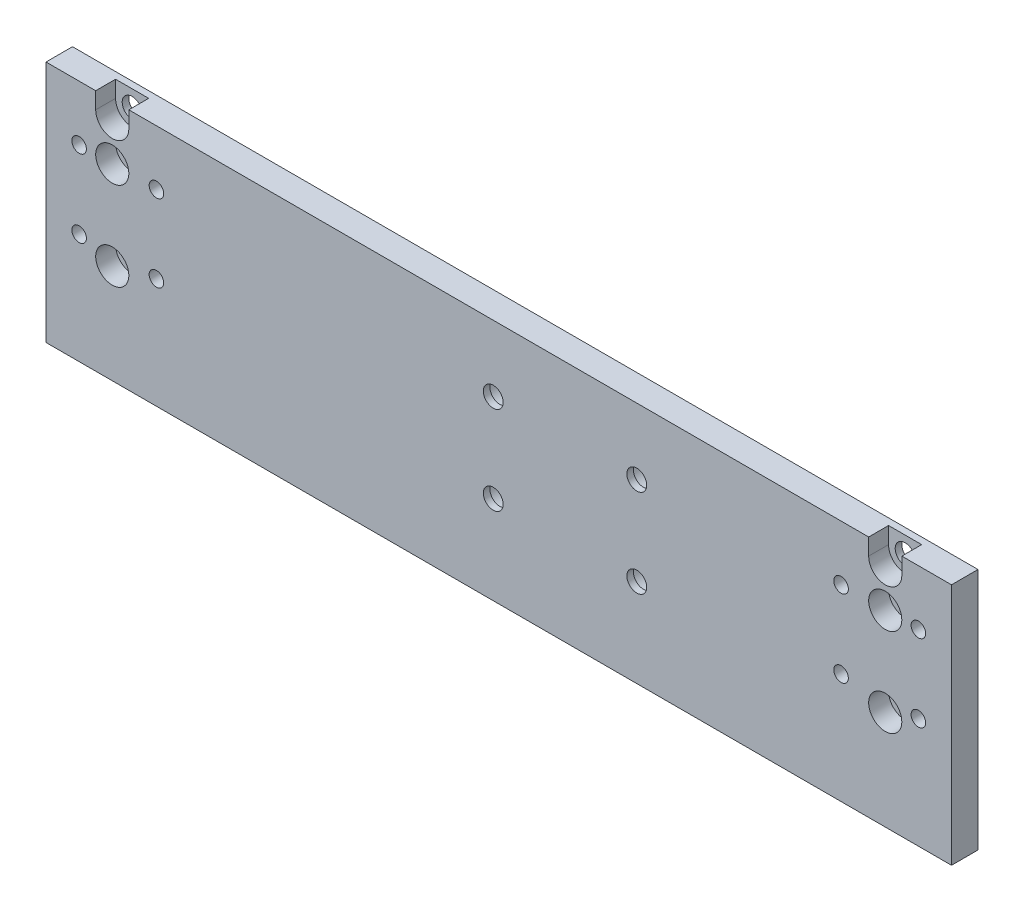
SolidWorks part; units mm, degrees
material "6061 合金"
ref_plane "前视基准面" through (0, 0, 0) normal (0, 0, 1) x (1, 0, 0)
ref_plane "上视基准面" through (0, 0, 0) normal (0, 1, 0) x (1, 0, 0)
ref_plane "右视基准面" through (0, 0, 0) normal (1, 0, 0) x (0, 0, -1)
sketch "草图1" plane through (0, 0, 0) normal (0, 0, 1) x (1, 0, 0)
  line L1 (-205, 55) -> (205, 55)
  line L2 (-205, 55) -> (-205, -55)
  line L3 (-205, -55) -> (205, -55)
  line L4 (205, 55) -> (205, -55)
  line L5 (-205, 55) -> (205, -55) construction
  line L6 (-205, -55) -> (205, 55) construction
  point P0 (0, 0)
  dimension "D1" = 410
  dimension "D2" = 110
extrude "凸台-拉伸1" add sketch "草图1" along normal mid plane 12
hole_wizard "打孔尺寸(%根据)内六角圆柱头螺钉的类型3" positions "3D草图1" profile "草图3" counterbore size "M6" standard "GB"
sketch3d "3D草图1"
  line L1 (205, -55, -6) -> (205, 55, -6) construction
  line L2 (205, 55, -6) -> (-205, 55, -6) construction
  point P0 (190, 30, -6)
  point P2 (155, 30, -6)
  point P4 (190, -5, -6)
  point P6 (155, -5, -6)
  dimension "D1" = 35
  dimension "D2" = 35
  dimension "D3" = 15
  dimension "D4" = 15
  dimension "D5" = 25
  dimension "D6" = 25
  dimension "D7" = 35
  dimension "D8" = 35
sketch "草图3" plane through (190, 30, -6) normal (1, 0, 0) x (0, 1, 0)
  line L0 (0, 0) -> (0, 14.3828)
  line L1 (0, 14.3828) -> (3.3, 12.4)
  line L2 (3.3, 12.4) -> (3.3, 6.8)
  line L3 (3.3, 6.8) -> (5.5, 6.8)
  line L4 (5.5, 6.8) -> (5.5, 0)
  line L5 (5.5, 0) -> (0, 0)
  line L10 (0, 14.3828) -> (-3.3, 12.4) construction
  line L11 (0, -6.35) -> (0, 107.95) construction
  dimension "孔直径" = 6.6
  dimension "孔深度" = 12.4
  dimension "柱形沉头孔直径" = 11
  dimension "柱形沉头孔深度" = 6.8
  dimension "导头角度" = 118
pattern_linear "阵列(线性)1" count 2 spacing 345 along (-1, 0, 0) of "打孔尺寸(%根据)内六角圆柱头螺钉的类型3"
hole_wizard "打孔尺寸(%根据)内六角圆柱头螺钉的类型2" positions "3D草图2" profile "草图4" counterbore size "M8" standard "GB"
sketch3d "3D草图2"
  line L0 (205, 55, -6) -> (-205, 55, -6) construction
  line L1 (-205, -55, -6) -> (205, -55, -6) construction
  line L2 (-205, 55, -6) -> (-205, -55, -6) construction
  point P0 (62.5, 25, -6)
  point P2 (62.5, -15, -6)
  point P4 (-2.5, -15, -6)
  point P6 (-2.5, 25, -6)
  dimension "D1" = 65
  dimension "D2" = 65
  dimension "D3" = 30
  dimension "D4" = 40
  dimension "D5" = 40
  dimension "D6" = 30
  dimension "D7" = 202.5
  dimension "D8" = 202.5
sketch "草图4" plane through (62.5, 25, -6) normal (1, 0, 0) x (0, 1, 0)
  line L0 (0, 0) -> (0, 15.1039)
  line L1 (0, 15.1039) -> (4.5, 12.4)
  line L2 (4.5, 12.4) -> (4.5, 9)
  line L3 (4.5, 9) -> (7.5, 9)
  line L4 (7.5, 9) -> (7.5, 0)
  line L5 (7.5, 0) -> (0, 0)
  line L10 (0, 15.1039) -> (-4.5, 12.4) construction
  line L11 (0, -6.35) -> (0, 107.95) construction
  dimension "孔直径" = 9
  dimension "孔深度" = 12.4
  dimension "柱形沉头孔直径" = 15
  dimension "柱形沉头孔深度" = 9
  dimension "导头角度" = 118
hole_wizard "打孔尺寸(%根据)内六角圆柱头螺钉的类型3" positions "3D草图3" profile "草图5" counterbore size "M8" standard "GB"
sketch3d "3D草图3"
  line L0 (-205, 55, 6) -> (-205, -55, 6) construction
  line L1 (205, 55, 6) -> (-205, 55, 6) construction
  point P4 (-175, 30, 6)
  point P6 (-175, -10, 6)
  dimension "D2" = 30
  dimension "D3" = 30
  dimension "D4" = 40
  dimension "D8" = 25
sketch "草图5" plane through (-175, 30, 6) normal (1, 0, 0) x (0, -1, 0)
  line L0 (0, 0) -> (0, 15.1039)
  line L1 (0, 15.1039) -> (4.5, 12.4)
  line L2 (4.5, 12.4) -> (4.5, 9)
  line L3 (4.5, 9) -> (7.5, 9)
  line L4 (7.5, 9) -> (7.5, 0)
  line L5 (7.5, 0) -> (0, 0)
  line L10 (0, 15.1039) -> (-4.5, 12.4) construction
  line L11 (0, -6.35) -> (0, 107.95) construction
  dimension "孔直径" = 9
  dimension "孔深度" = 12.4
  dimension "柱形沉头孔直径" = 15
  dimension "柱形沉头孔深度" = 9
  dimension "导头角度" = 118
sketch "草图14" plane through (0, 0, 6) normal (0, 0, 1) x (1, 0, 0)
  line L0 (205, 55) -> (-205, 55) construction
  line L1 (-205, 55) -> (-205, -55) construction
  circle A0 centre (-175, 47.5) radius 4.5
  dimension "D1" = 9
  dimension "D2" = 7.5
  dimension "D3" = 30
extrude "切除-拉伸1" cut sketch "草图14" against normal through all contours A0
sketch "草图15" plane through (0, 0, 6) normal (0, 0, 1) x (1, 0, 0)
  line L0 (-175, 47.5) -> (-175, 101.2893) construction
  line L1 (-182.5, 47.5) -> (-182.5, 101.2893)
  line L2 (-167.5, 47.5) -> (-167.5, 101.2893)
  arc A0 (-182.5, 47.5) -> (-167.5, 47.5) centre (-175, 47.5) ccw
  arc A1 (-167.5, 101.2893) -> (-182.5, 101.2893) centre (-175, 101.2893) ccw
  point P3 (-175, 74.3947)
  dimension "D1" = 15
extrude "切除-拉伸2" cut sketch "草图15" against normal blind 9 contours L1 A1 L2 A0
pattern_linear "阵列(线性)2" count 2 spacing 350 along (1, 0, 0) of "切除-拉伸2", "打孔尺寸(%根据)内六角圆柱头螺钉的类型3", "切除-拉伸1"
